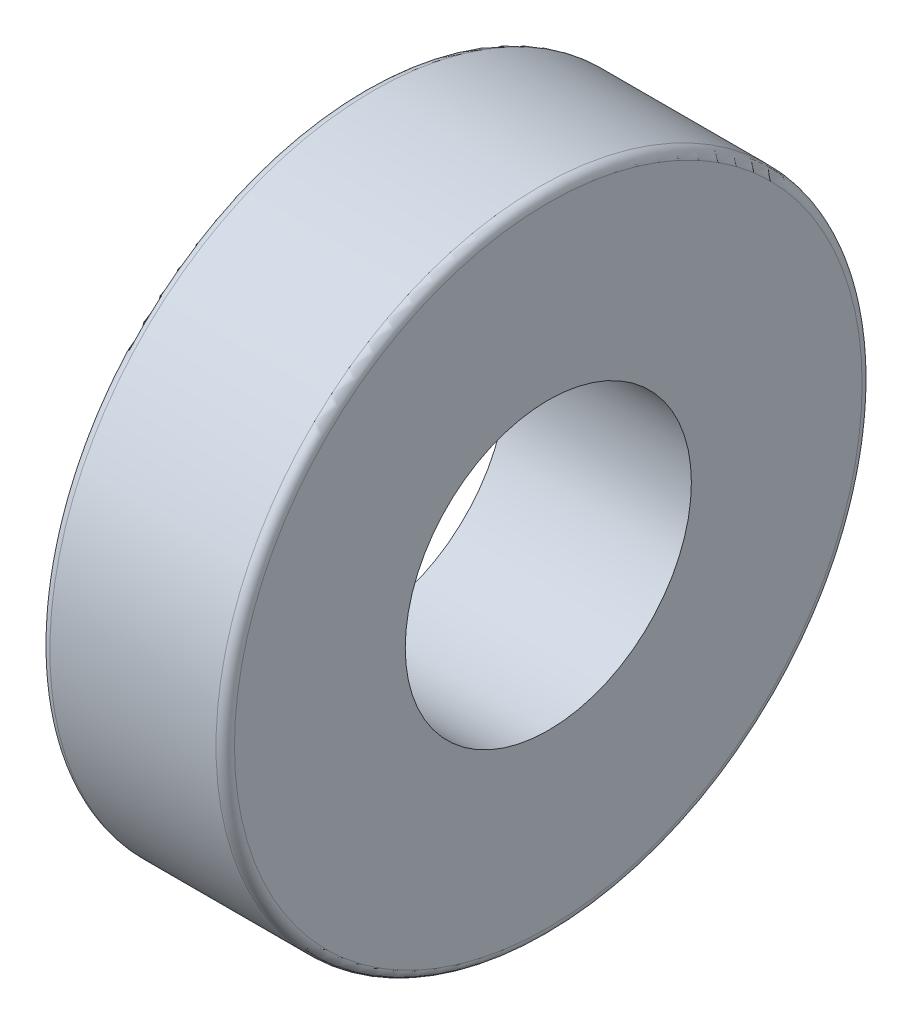
from build123d import *

# Parameters (mm, degrees)
SKETCH_1_W          = 40
SKETCH_1_H          = 70
SKETCH_2_R          = 31
CUT_EXTRUDE_1_DEPTH = 107.77078252
FILLET_1_R          = 2


with BuildPart() as part:
    # 草图1 → 旋转1 (revolve)
    with BuildSketch(Plane.XY, mode=Mode.PRIVATE) as revolve_1_sk:
        with Locations((0, 35)):
            Rectangle(SKETCH_1_W, SKETCH_1_H)
    revolve(revolve_1_sk.sketch.rotate(Axis((-20, 0, 0), (1, 0, 0)), 180), axis=Axis((-20, 0, 0), (1, 0, 0)))

    # 草图2 → 切除-拉伸1 (cut, through all)
    with BuildSketch(Plane(origin=(20, 0, 0), x_dir=(0, 0, -1), z_dir=(1, 0, 0))):
        with Locations(Location((0, 0, 0), (0, 0, 90))):
            Circle(SKETCH_2_R)
    extrude(amount=-CUT_EXTRUDE_1_DEPTH, mode=Mode.SUBTRACT)

    # 圆角1
    fillet_1_edges = [part.edges().sort_by_distance(p)[0] for p in [
        (-20, 70, 0),
        (20, 70, 0),
    ]]
    fillet(fillet_1_edges, radius=FILLET_1_R)


solid = part.part
